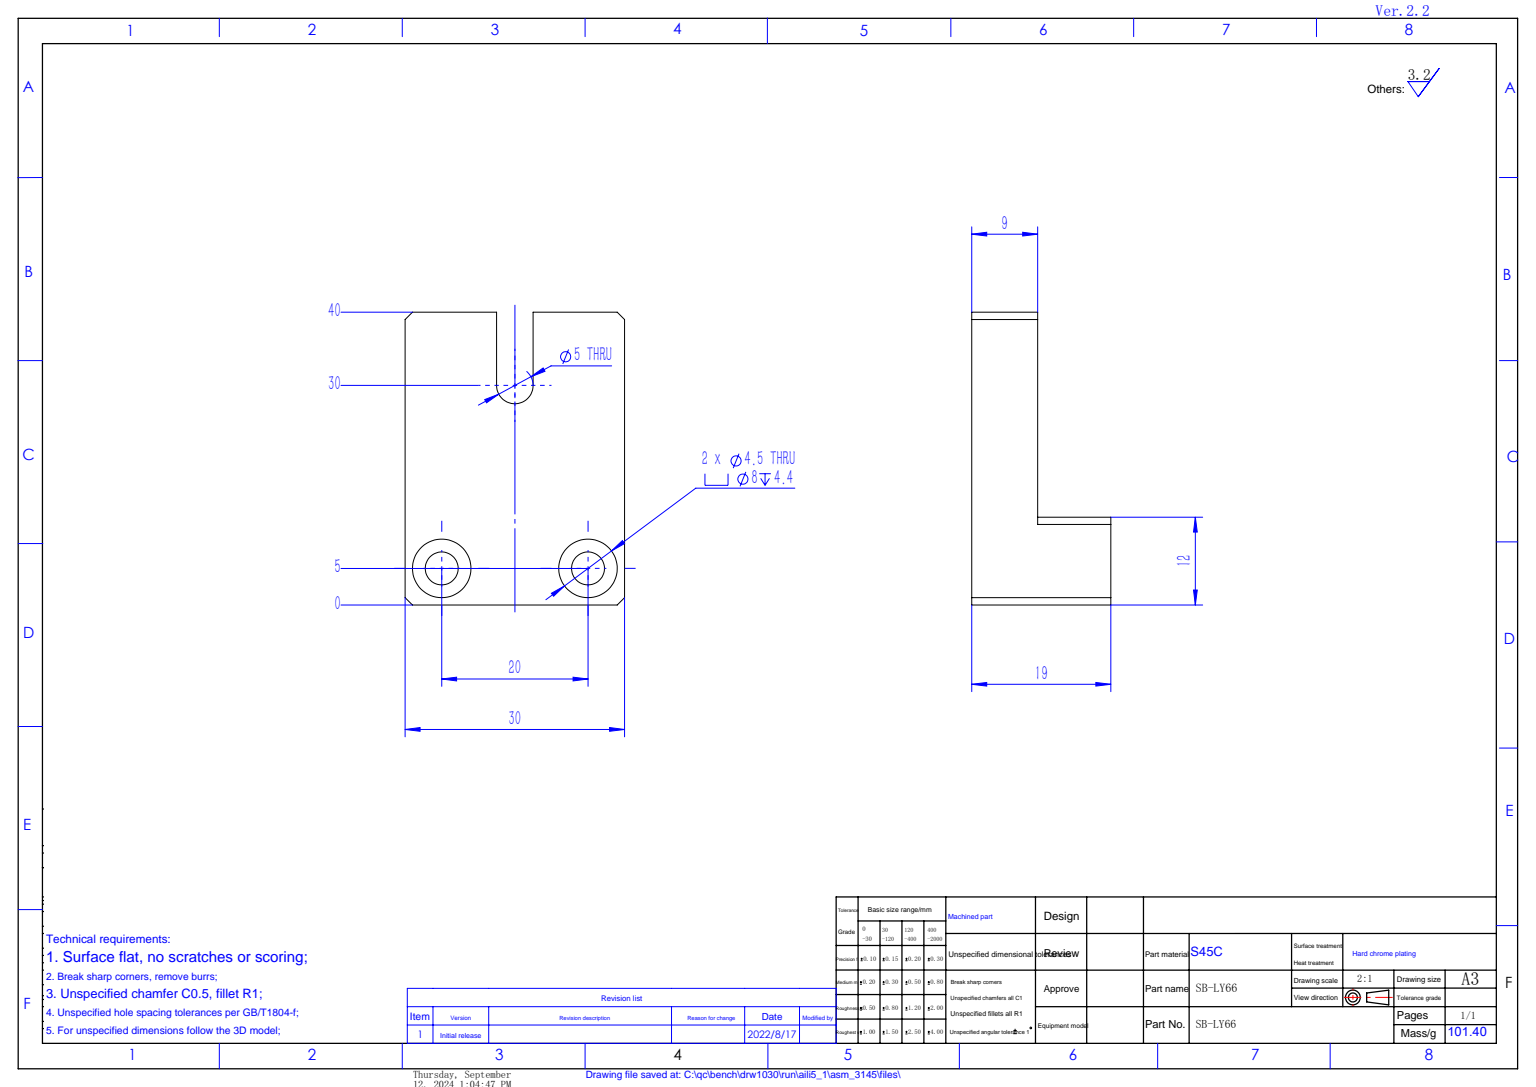
from build123d import *

# Parameters (mm, degrees)
SKETCH_1_W                   = 30
SKETCH_1_H                   = 40
EXTRUDE_1_DEPTH              = 9
SKETCH_2_W                   = 30
SKETCH_2_H                   = 12
EXTRUDE_2_DEPTH              = 10
HOLE_WIZARD_M4_1_D           = 4.5
HOLE_WIZARD_M4_1_CBORE_D     = 8
HOLE_WIZARD_M4_1_CBORE_DEPTH = 4.4
CHAMFER_1_SIZE               = 1
CUT_EXTRUDE_1_DEPTH          = 32.400636936


with BuildPart() as part:
    # 草图1 → 凸台-拉伸1 (new body)
    with BuildSketch(Plane(origin=(0, 0, 0), x_dir=(1, 0, 0), z_dir=(0, 1, 0))):
        Rectangle(SKETCH_1_W, SKETCH_1_H)
    extrude(amount=EXTRUDE_1_DEPTH)

    # 草图2 → 凸台-拉伸2 (add)
    with BuildSketch(Plane(origin=(0, 9, 0), x_dir=(1, 0, 0), z_dir=(0, 1, 0))):
        with Locations((0, 14)):
            Rectangle(SKETCH_2_W, SKETCH_2_H)
    extrude(amount=EXTRUDE_2_DEPTH)

    # M4 六角凹头螺钉的柱形沉头孔1 (through all)
    with Locations(Plane(origin=(0, 0, 0), x_dir=(-1, 0, 0), z_dir=(0, -1, 0))):
        with Locations((-10, 15), (10, 15)):
            CounterBoreHole(HOLE_WIZARD_M4_1_D / 2, HOLE_WIZARD_M4_1_CBORE_D / 2, HOLE_WIZARD_M4_1_CBORE_DEPTH)

    # 倒角1
    chamfer_1_edges = [part.edges().sort_by_distance(p)[0] for p in [
        (-15, 14, -8),
        (15, 14, -8),
        (-15, 9.5, -20),
        (15, 9.5, -20),
        (15, 4.5, 20),
        (-15, 4.5, 20),
    ]]
    chamfer(chamfer_1_edges, length=CHAMFER_1_SIZE)

    # 草图5 → 切除-拉伸1 (cut, through all)
    with BuildSketch(Plane.XZ):
        with BuildLine():
            Line((2.5, 20), (2.5, 10))
            ThreePointArc((2.5, 10), (0, 7.5), (-2.5, 10))
            Line((-2.5, 10), (-2.5, 20))
            ThreePointArc((-2.5, 20), (0, 22.5), (2.5, 20))
        make_face()
    extrude(amount=-CUT_EXTRUDE_1_DEPTH, mode=Mode.SUBTRACT)


solid = part.part
